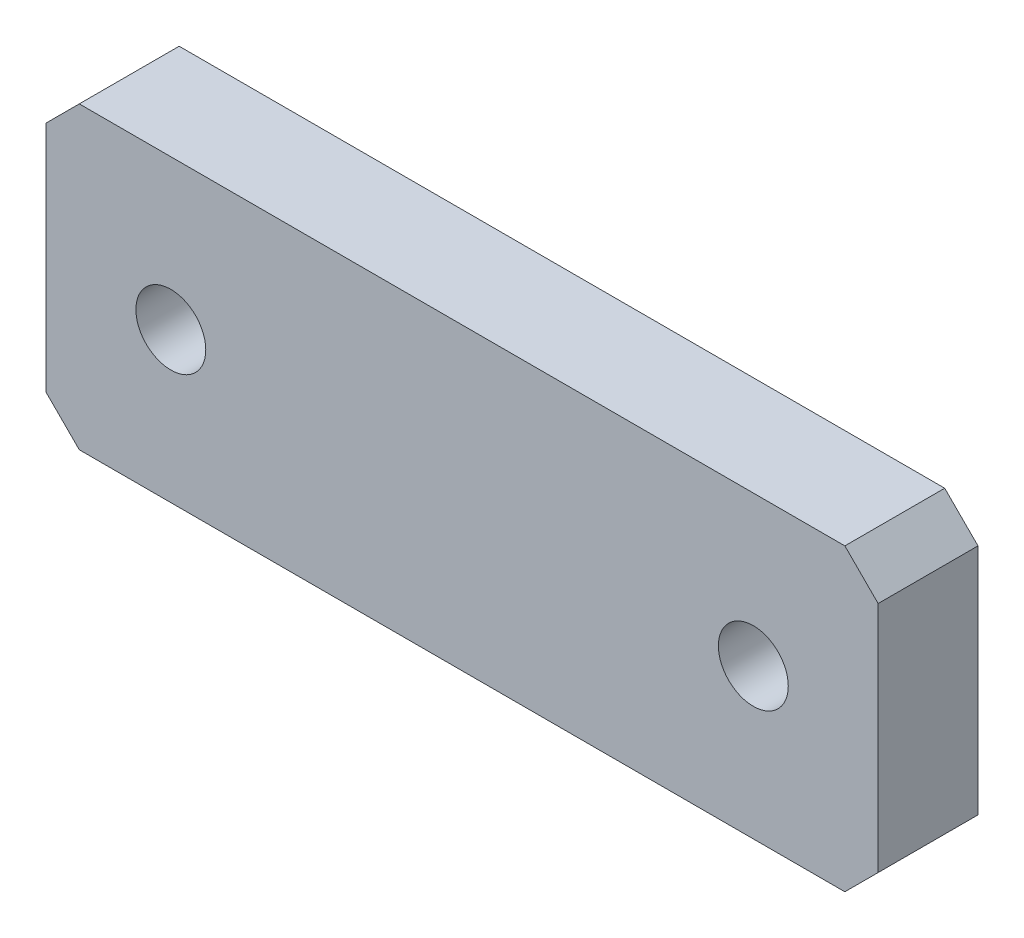
SolidWorks part; units mm, degrees
material "A5052"
ref_plane "Front Plane" through (0, 0, 0) normal (0, 0, 1) x (1, 0, 0)
ref_plane "Top Plane" through (0, 0, 0) normal (0, 1, 0) x (1, 0, 0)
ref_plane "Right Plane" through (0, 0, 0) normal (1, 0, 0) x (0, 0, -1)
sketch "Sketch1" plane through (0, 0, 0) normal (0, 0, 1) x (1, 0, 0)
  line L1 (25, -9) -> (-25, -9)
  line L2 (25, -9) -> (25, 9)
  line L3 (25, 9) -> (-25, 9)
  line L4 (-25, -9) -> (-25, 9)
  line L5 (25, -9) -> (-25, 9) construction
  line L6 (25, 9) -> (-25, -9) construction
  point P0 (0, 0)
  dimension "D1" = 18
  dimension "D2" = 50
extrude "Boss-Extrude1" add sketch "Sketch1" along normal mid plane 6
hole_wizard "M5 Tapped Hole1" positions "Sketch2" profile "Sketch3" tap size "M5" standard "GB" end condition through all
sketch "Sketch2" plane through (0, 0, 3) normal (0, 0, 1) x (1, 0, 0)
  point P0 (-17.5, 0)
  point P3 (17.5, 0)
sketch "Sketch3" plane through (-17.5, 0, 3) normal (1, 0, 0) x (0, -1, 0)
  line L0 (0, 0) -> (0, 6)
  line L1 (0, 6) -> (2.1, 6)
  line L2 (2.1, 6) -> (2.1, 0)
  line L5 (2.1, 0) -> (0, 0)
  line L11 (0, -6.35) -> (0, 107.95) construction
  dimension "通孔螺纹孔钻头直径" = 4.2
  dimension "通孔螺纹孔钻头深度" = 6
cosmetic thread "Hole thread 1" parameters "D2"=5
cosmetic thread "Hole thread 2" parameters "D2"=5
chamfer "Chamfer1" distance 2 angle 45 4 edges at (25, 9, 0) (25, -9, 0) (-25, -9, 0) (-25, 9, 0)
